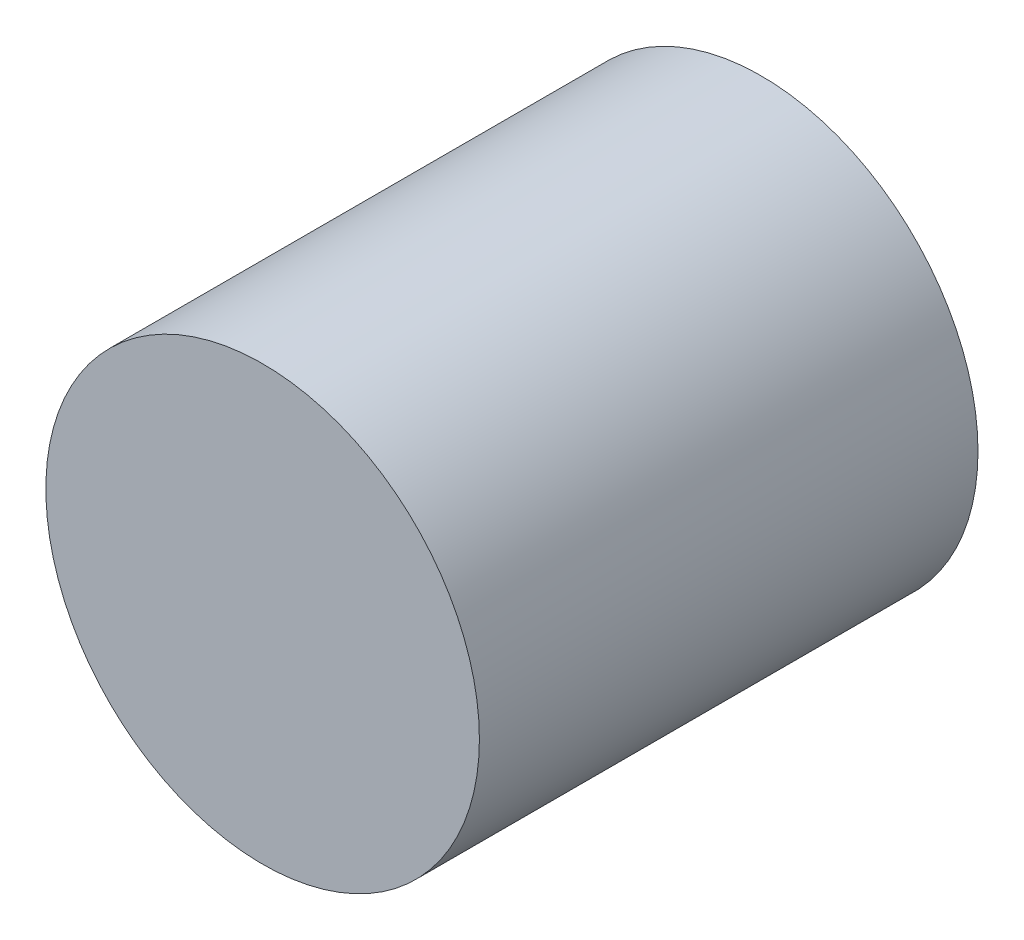
SolidWorks part; units mm, degrees
ref_plane "Front Plane" through (0, 0, 0) normal (0, 0, 1) x (1, 0, 0)
ref_plane "Top Plane" through (0, 0, 0) normal (0, 1, 0) x (1, 0, 0)
ref_plane "Right Plane" through (0, 0, 0) normal (1, 0, 0) x (0, 0, -1)
other "Configuration Table"
sketch "Sketch2" plane through (0, 0, 0) normal (0, 0, 1) x (1, 0, 0)
  circle A0 centre (121.6742, 138.644) radius 20
  dimension "D1" = 40
extrude "Boss-Extrude1" add sketch "Sketch2" along normal blind 46
